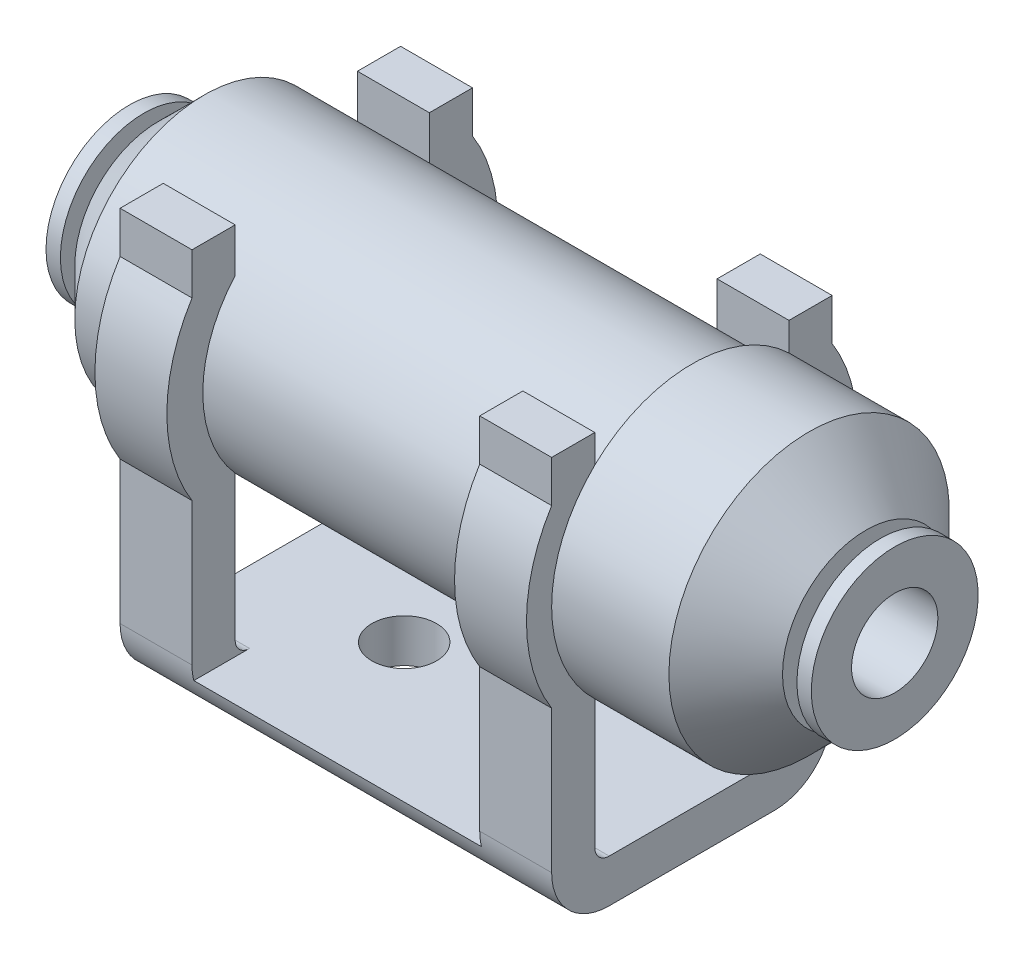
from build123d import *

# Parameters (mm, degrees)
EXTRUDE_1_DEPTH     = 5
EXTRUDE_START       = -5
EXTRUDE_2_DEPTH     = 5
EXTRUDE_3_DEPTH     = 15
EXTRUDE_4_DEPTH     = 5
SKETCH_6_R          = 2.25
CUT_EXTRUDE_1_DEPTH = 4
SKETCH_7_R          = 2.25
CUT_EXTRUDE_2_DEPTH = 4
SKETCH_8_R          = 3
CUT_EXTRUDE_3_DEPTH = 24.1
CUT_EXTRUDE_START   = -19.1
SKETCH_9_R          = 3
CUT_EXTRUDE_4_DEPTH = 19.1


with BuildPart() as part:
    # 草图1 → 旋转1 (revolve)
    with BuildSketch(Plane.XY, mode=Mode.PRIVATE) as revolve_1_sk:
        Polygon((-19.1, 20), (-19.1, 25.8), (-18.1, 25.8), (-18.1, 24), (-17.1, 24), (-17.1, 25.8), (-13.9, 29), (20, 29), (20, 29.75), (28.15, 29.75), (32.1, 25.8), (32.1, 24), (33.1, 24), (33.1, 25.8), (34.1, 25.8), (34.1, 20), align=None)
    revolve(revolve_1_sk.sketch.rotate(Axis((34.1, 20, 0), (-1, 0, 0)), 270), axis=Axis((34.1, 20, 0), (-1, 0, 0)))

    # 草图2 → 凸台-拉伸1 (add)
    with BuildSketch(Plane(origin=(-10, 0, 0), x_dir=(0, 0, -1), z_dir=(1, 0, 0))):
        with BuildLine():
            Line((-9.75, 13.901844541), (-9.75, 4))
            ThreePointArc((-9.75, 4), (-8.578427125, 1.171572875), (-5.75, 0))
            Line((-5.75, 0), (5.75, 0))
            ThreePointArc((5.75, 0), (8.578427125, 1.171572875), (9.75, 4))
            Line((9.75, 4), (9.75, 13.901844541))
            ThreePointArc((9.75, 13.901844541), (11.5, 20), (9.75, 26.098155459))
            Line((9.75, 26.098155459), (9.75, 29))
            Line((9.75, 29), (6.75, 29))
            Line((6.75, 29), (6.75, 22))
            Line((6.75, 22), (-6.75, 22))
            Line((-6.75, 22), (-6.75, 29))
            Line((-6.75, 29), (-9.75, 29))
            Line((-9.75, 29), (-9.75, 26.098155459))
            ThreePointArc((-9.75, 26.098155459), (-11.5, 20), (-9.75, 13.901844541))
        make_face()
        with BuildLine():
            Line((-5.75, 3), (5.75, 3))
            ThreePointArc((5.75, 3), (6.457106781, 3.292893219), (6.75, 4))
            Line((6.75, 4), (6.75, 20))
            Line((6.75, 20), (-6.75, 20))
            Line((-6.75, 20), (-6.75, 4))
            ThreePointArc((-6.75, 4), (-6.457106781, 3.292893219), (-5.75, 3))
        make_face(mode=Mode.SUBTRACT)
    extrude(amount=EXTRUDE_1_DEPTH)

    # 草图3 → 凸台-拉伸2 (add)
    with BuildSketch(Plane(origin=(20, 0, 0), x_dir=(0, 0, -1), z_dir=(1, 0, 0)).offset(EXTRUDE_START)):
        with BuildLine():
            Line((-9.75, 13.901844541), (-9.75, 4))
            ThreePointArc((-9.75, 4), (-8.578427125, 1.171572875), (-5.75, 0))
            Line((-5.75, 0), (5.75, 0))
            ThreePointArc((5.75, 0), (8.578427125, 1.171572875), (9.75, 4))
            Line((9.75, 4), (9.75, 13.901844541))
            ThreePointArc((9.75, 13.901844541), (11.5, 20), (9.75, 26.098155459))
            Line((9.75, 26.098155459), (9.75, 29))
            Line((9.75, 29), (6.75, 29))
            Line((6.75, 29), (6.75, 22))
            Line((6.75, 22), (-6.75, 22))
            Line((-6.75, 22), (-6.75, 29))
            Line((-6.75, 29), (-9.75, 29))
            Line((-9.75, 29), (-9.75, 26.098155459))
            ThreePointArc((-9.75, 26.098155459), (-11.5, 20), (-9.75, 13.901844541))
        make_face()
        with BuildLine():
            Line((-5.75, 3), (5.75, 3))
            ThreePointArc((5.75, 3), (6.457106781, 3.292893219), (6.75, 4))
            Line((6.75, 4), (6.75, 20))
            Line((6.75, 20), (-6.75, 20))
            Line((-6.75, 20), (-6.75, 4))
            ThreePointArc((-6.75, 4), (-6.457106781, 3.292893219), (-5.75, 3))
        make_face(mode=Mode.SUBTRACT)
    extrude(amount=EXTRUDE_2_DEPTH)

    # 草图4 → 凸台-拉伸3 (add)
    with BuildSketch(Plane(origin=(0, 0, 0), x_dir=(0, 0, -1), z_dir=(1, 0, 0))):
        with BuildLine():
            Line((-5.75, 0), (5.75, 0))
            ThreePointArc((5.75, 0), (8.199489743, 0.83772234), (9.622983346, 3))
            Line((9.622983346, 3), (-9.622983346, 3))
            ThreePointArc((-9.622983346, 3), (-8.199489743, 0.83772234), (-5.75, 0))
        make_face()
    extrude(amount=EXTRUDE_3_DEPTH)

    # 草图5 → 凸台-拉伸4 (add)
    with BuildSketch(Plane(origin=(0, 0, 0), x_dir=(0, 0, -1), z_dir=(1, 0, 0)).offset(EXTRUDE_START)):
        with BuildLine():
            Line((-5.75, 0), (5.75, 0))
            ThreePointArc((5.75, 0), (8.199489743, 0.83772234), (9.622983346, 3))
            Line((9.622983346, 3), (-9.622983346, 3))
            ThreePointArc((-9.622983346, 3), (-8.199489743, 0.83772234), (-5.75, 0))
        make_face()
    extrude(amount=EXTRUDE_4_DEPTH)

    # 草图6 → 切除-拉伸1 (cut)
    with BuildSketch(Plane(origin=(0, 0, 0), x_dir=(1, 0, 0), z_dir=(0, 1, 0))):
        with Locations(Location((0, 0, 0), (0, 0, 270))):
            Circle(SKETCH_6_R)
    extrude(amount=CUT_EXTRUDE_1_DEPTH, mode=Mode.SUBTRACT)

    # 草图7 → 切除-拉伸2 (cut)
    with BuildSketch(Plane(origin=(0, 0, 0), x_dir=(1, 0, 0), z_dir=(0, 1, 0))):
        with Locations(Location((10, 0, 0), (0, 0, 270))):
            Circle(SKETCH_7_R)
    extrude(amount=CUT_EXTRUDE_2_DEPTH, mode=Mode.SUBTRACT)

    # 草图8 → 切除-拉伸3 (cut)
    with BuildSketch(Plane(origin=(34.1, 0, 0), x_dir=(0, 0, -1), z_dir=(1, 0, 0))):
        with Locations((0, 20)):
            Circle(SKETCH_8_R)
    extrude(amount=-CUT_EXTRUDE_3_DEPTH, mode=Mode.SUBTRACT)

    # 草图9 → 切除-拉伸4 (cut)
    with BuildSketch(Plane.ZY.offset(19.1).offset(CUT_EXTRUDE_START)):
        with Locations(Location((0, 20, 0), (0, 0, 180))):
            Circle(SKETCH_9_R)
    extrude(amount=CUT_EXTRUDE_4_DEPTH, mode=Mode.SUBTRACT)


solid = part.part
